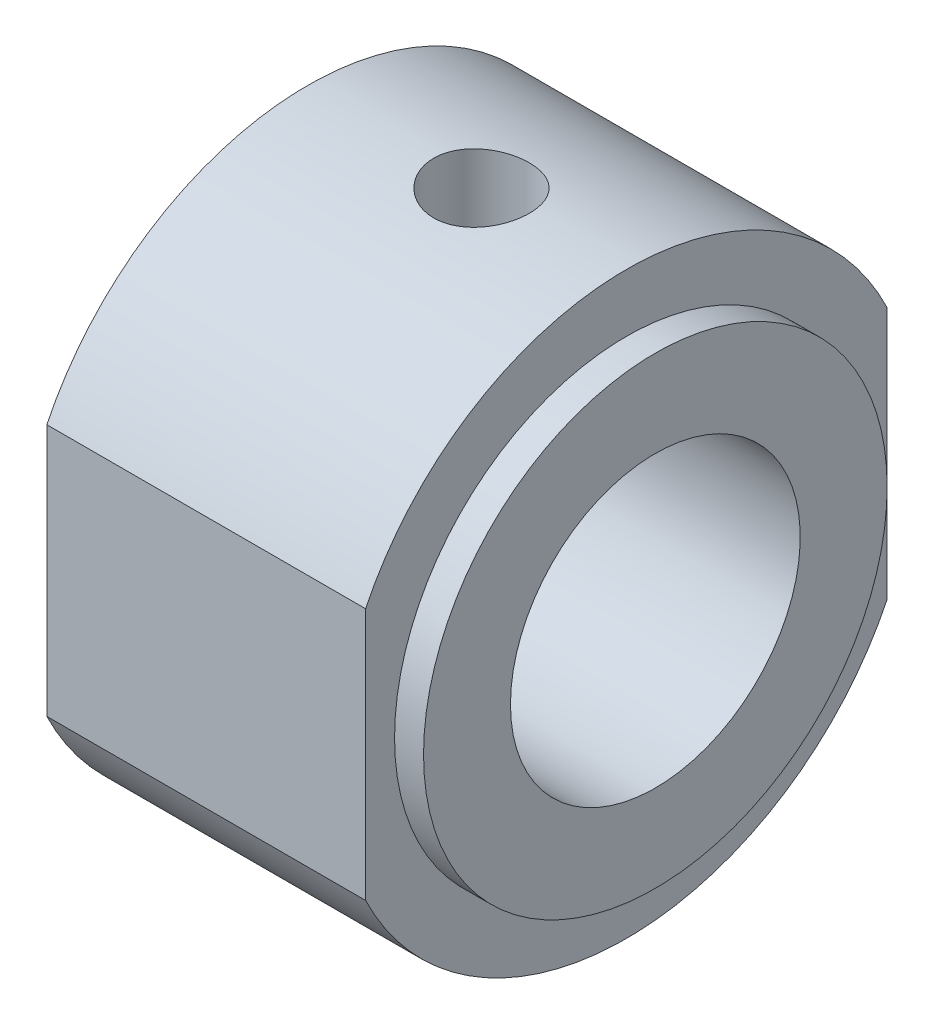
SolidWorks part; units mm, degrees
ref_plane "Front Plane" through (0, 0, 0) normal (0, 0, 1) x (1, 0, 0)
ref_plane "Top Plane" through (0, 0, 0) normal (0, 1, 0) x (1, 0, 0)
ref_plane "Right Plane" through (0, 0, 0) normal (1, 0, 0) x (0, 0, -1)
sketch "Sketch1" plane through (0, 0, 0) normal (0, 0, 1) x (1, 0, 0)
  line L0 (0, 0) -> (51.1502, 0) construction
  line L1 (0, 5) -> (0, 10)
  line L2 (0, 10) -> (11, 10)
  line L3 (11, 10) -> (11, 8)
  line L4 (11, 8) -> (12, 8)
  line L5 (12, 8) -> (12, 5)
  line L6 (12, 5) -> (0, 5)
  dimension "D1" = 12
  dimension "D2" = 1
  dimension "D3" = 10
  dimension "D4" = 5
  dimension "D5" = 8
revolve "Revolve1" add sketch "Sketch1" angle 360 about L0
cosmetic thread "Cosmetic Thread1" parameters "D2"=12
sketch "Sketch2" plane through (0, 0, 0) normal (-1, 0, 0) x (0, 0, 1)
  line L1 (-9, 12.5) -> (9, 12.5)
  line L2 (-9, 12.5) -> (-9, -12.5)
  line L3 (-9, -12.5) -> (9, -12.5)
  line L4 (9, 12.5) -> (9, -12.5)
  line L5 (-9, 12.5) -> (9, -12.5) construction
  line L6 (-9, -12.5) -> (9, 12.5) construction
  point P0 (0, 0)
  dimension "D1" = 18
  dimension "D2" = 25
extrude "Cut-Extrude1" cut sketch "Sketch2" against normal through all flip side to cut
ref_plane "Plane1" through (0, 10, 0) normal (0, 1, 0) x (-1, 0, 0)
hole_wizard "M4 Tapped Hole1" positions "Sketch4" profile "Sketch3" tap size "M4" standard "GB"
sketch "Sketch4" plane through (0, 10, 0) normal (0, 1, 0) x (-1, 0, 0)
  point P1 (-6, 0)
  dimension "D1" = 6
cosmetic thread "孔螺蚊线1" parameters "D2"=4
sketch "Sketch3" plane through (6, 10, 0) normal (1, 0, 0) x (0, 0, 1)
  line L0 (0, 0) -> (0, 5)
  line L1 (0, 5) -> (1.65, 5)
  line L2 (1.65, 5) -> (1.65, 0)
  line L5 (1.65, 0) -> (0, 0)
  line L11 (0, -6.35) -> (0, 107.95) construction
  dimension "通孔螺纹孔钻头直径" = 3.3
  dimension "通孔螺纹孔钻头深度" = 5
